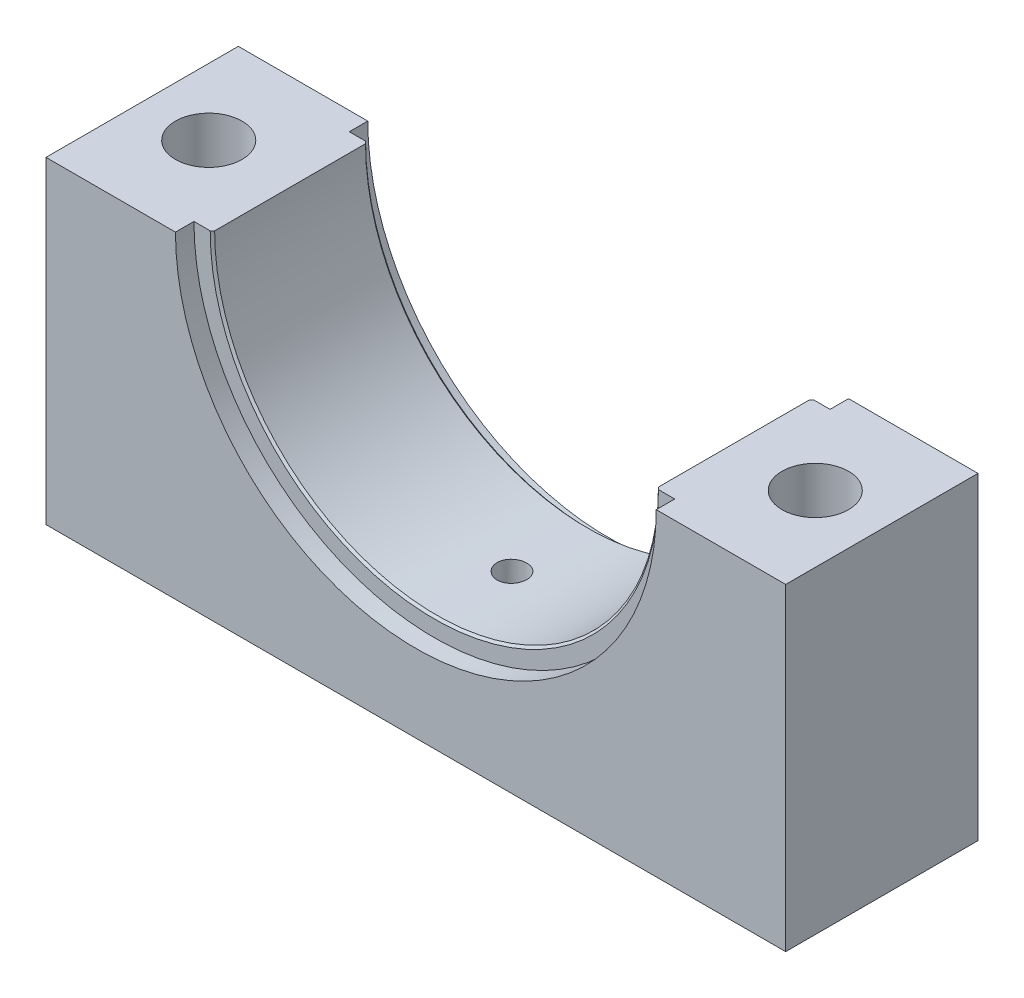
SolidWorks part; units mm, degrees
material "Q235-A"
ref_plane "Front Plane" through (0, 0, 0) normal (0, 0, 1) x (1, 0, 0)
ref_plane "Top Plane" through (0, 0, 0) normal (0, 1, 0) x (1, 0, 0)
ref_plane "Right Plane" through (0, 0, 0) normal (1, 0, 0) x (0, 0, -1)
sketch "Sketch1" plane through (0, 0, 0) normal (0, 0, 1) x (1, 0, 0)
  line L0 (-50, 0) -> (-30, 0)
  line L1 (-50, -43) -> (50, -43)
  line L2 (-50, -43) -> (-50, 0)
  line L4 (50, -43) -> (50, 0)
  line L5 (-50, -43) -> (0, 0) construction
  line L6 (22.7456, -19.5612) -> (50, -43) construction
  line L7 (30, 0) -> (50, 0)
  arc A0 (-30, 0) -> (30, 0) centre (0, 0) ccw
  point P0 (0, 0)
  dimension "D1" = 43
  dimension "D2" = 100
extrude "Boss-Extrude1" add sketch "Sketch1" along normal blind 26
sketch "Sketch2" plane through (0, 0, 26) normal (0, 0, 1) x (1, 0, 0)
  circle A0 centre (0, 0) radius 32.5
extrude "Cut-Extrude1" cut sketch "Sketch2" against normal blind 2.5
sketch "Sketch3" plane through (0, 0, 0) normal (0, 0, -1) x (-1, 0, 0)
  circle A1 centre (0, 0) radius 32.5
  circle A2 centre (0, 0) radius 32.5
  dimension "D1" = 0
extrude "Cut-Extrude2" cut sketch "Sketch3" against normal blind 2.5
chamfer "Chamfer1" distance 0.3 angle 45 2 edges at (0, -30, 2.5) (0, -30, 23.5)
sketch "Sketch4" plane through (0, 0, 0) normal (0, 1, 0) x (1, 0, 0)
  line L0 (-41, -13) -> (41, -13)
  line L1 (-50, -26) -> (-50, 0) construction
  dimension "D1" = 82
  dimension "D2" = 9
hole_wizard "Hole1" positions "Sketch5" profile "Sketch6" legacy end condition through all
sketch "Sketch5" plane through (0, 0, 0) normal (0, 1, 0) x (1, 0, 0)
  point P0 (-41, -13)
  point P3 (41, -13)
sketch "Sketch6" plane through (-41, 0, 13) normal (1, 0, 0) x (0, 0, 1)
  line L0 (0, 0) -> (0, 43)
  line L1 (0, 43) -> (4.5, 43)
  line L2 (4.5, 43) -> (4.5, 0)
  line L3 (4.5, 0) -> (0, 0)
  line L4 (0, 110) -> (0, -10) construction
  dimension "直径" = 9
  dimension "深度" = 43
sketch "Sketch8" plane through (0, 0, 0) normal (0, 1, 0) x (1, 0, 0)
  line L0 (0, -26) -> (0, 0)
  line L1 (-32.5, -26) -> (32.5, -26) construction
  line L2 (32.5, 0) -> (-32.5, 0) construction
hole_wizard "Hole2" positions "Sketch9" profile "Sketch10" legacy
sketch "Sketch9" plane through (0, 0, 0) normal (0, 1, 0) x (1, 0, 0)
  line L0 (0, -26) -> (0, 0) construction
  point P0 (0, -13)
sketch "Sketch10" plane through (0, 0, 13) normal (1, 0, 0) x (0, 0, 1)
  line L0 (0, 0) -> (0, 34)
  line L1 (0, 34) -> (2, 34)
  line L2 (2, 34) -> (2, 0)
  line L3 (2, 0) -> (0, 0)
  line L4 (0, 110) -> (0, -10) construction
  dimension "直径" = 4
  dimension "深度" = 34
sketch "Sketch11" plane through (0, -43, 0) normal (0, -1, 0) x (1, 0, 0)
  line L0 (21, 0) -> (21, 26)
  line L1 (-50, 0) -> (50, 0) construction
  line L2 (-50, 26) -> (50, 26) construction
  line L4 (-50, 13) -> (-4.2128, 13) construction
  line L5 (-50, 26) -> (-50, 0) construction
  line L6 (-20, 13) -> (-22, 13) construction
  line L7 (-20, 9) -> (-22, 9)
  line L8 (-20, 17) -> (-22, 17)
  arc A0 (-20, 9) -> (-20, 17) centre (-20, 13) ccw
  arc A1 (-22, 17) -> (-22, 9) centre (-22, 13) ccw
  point P13 (-21, 13)
  dimension "D3" = 4
  dimension "D1" = 21
  dimension "D2" = 2
  dimension "D4" = 41
hole_wizard "Hole4" positions "Sketch14" profile "Sketch15" legacy
sketch "Sketch14" plane through (0, -43, 0) normal (0, -1, 0) x (-1, 0, 0)
  line L0 (-21, 0) -> (-21, -26) construction
  point P0 (-21, -13)
sketch "Sketch15" plane through (21, -43, 13) normal (1, 0, 0) x (0, 0, -1)
  line L0 (0, 0) -> (0, 6)
  line L1 (0, 6) -> (4, 6)
  line L2 (4, 6) -> (4, 0)
  line L3 (4, 0) -> (0, 0)
  line L4 (0, 110) -> (0, -10) construction
  dimension "直径" = 8
  dimension "深度" = 6
extrude "Cut-Extrude4" cut sketch "Sketch11" against normal blind 6 contours L8 A1 L7 A0
